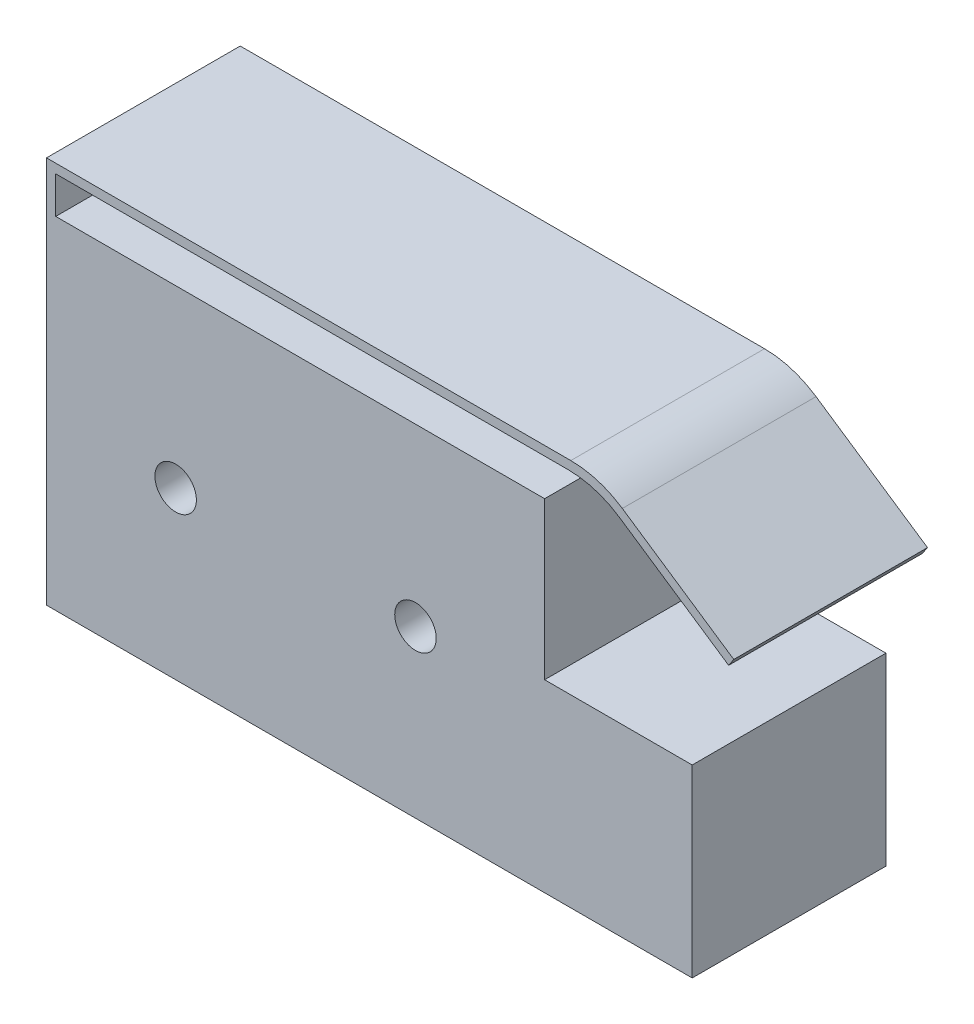
from build123d import *

# Parameters (mm, degrees)
SKETCH_1_R      = 2.25
EXTRUDE_1_DEPTH = 21
EXTRUDE_3_DEPTH = 21


with BuildPart() as part:
    # 草图1 → 凸台-拉伸1 (new body)
    with BuildSketch(Plane.XY):
        Polygon((0, 0), (70, 0), (70, 20), (54, 20), (54, 37), (0, 37), align=None)
        with Locations(Location((14, 18, 0), (0, 0, 180))):
            Circle(SKETCH_1_R, mode=Mode.SUBTRACT)
        with Locations(Location((40, 18, 0), (0, 0, 180))):
            Circle(SKETCH_1_R, mode=Mode.SUBTRACT)
    extrude(amount=EXTRUDE_1_DEPTH)

    # 草图2 → 凸台-拉伸3 (add)
    with BuildSketch(Plane.XY.offset(21)):
        with BuildLine():
            Line((62.423710356, 40.295115228), (74.506235043, 32.160250075))
            Line((74.506235043, 32.160250075), (73.947745443, 31.330738552))
            Line((73.947745443, 31.330738552), (62.118443298, 39.295115228))
            ThreePointArc((62.118443298, 39.295115228), (59.453208897, 40.564286494), (56.533547297, 41))
            Line((56.533547297, 41), (1, 41))
            Line((1, 41), (1, 37))
            Line((1, 37), (0, 37))
            Line((0, 37), (0, 42))
            Line((0, 42), (56.838814355, 42))
            ThreePointArc((56.838814355, 42), (59.758475955, 41.564286494), (62.423710356, 40.295115228))
        make_face()
    extrude(amount=-EXTRUDE_3_DEPTH)


solid = part.part
